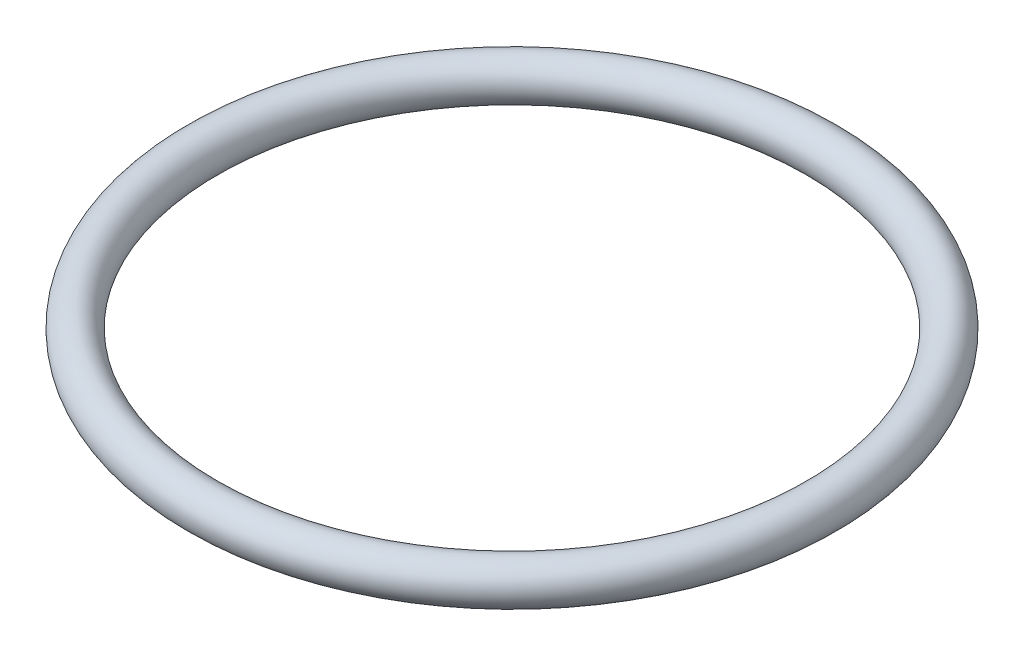
from build123d import *

# Parameters (mm, degrees)
SKETCH_1_R = 0.75


with BuildPart() as part:
    # 草图1 → 旋转1 (revolve)
    with BuildSketch(Plane.XY, mode=Mode.PRIVATE) as revolve_1_sk:
        with Locations((-11.25, 0)):
            Circle(SKETCH_1_R)
    revolve(revolve_1_sk.sketch.rotate(Axis((0, 0, 0), (0, 1, 0)), 270), axis=Axis((0, 0, 0), (0, 1, 0)))


solid = part.part
